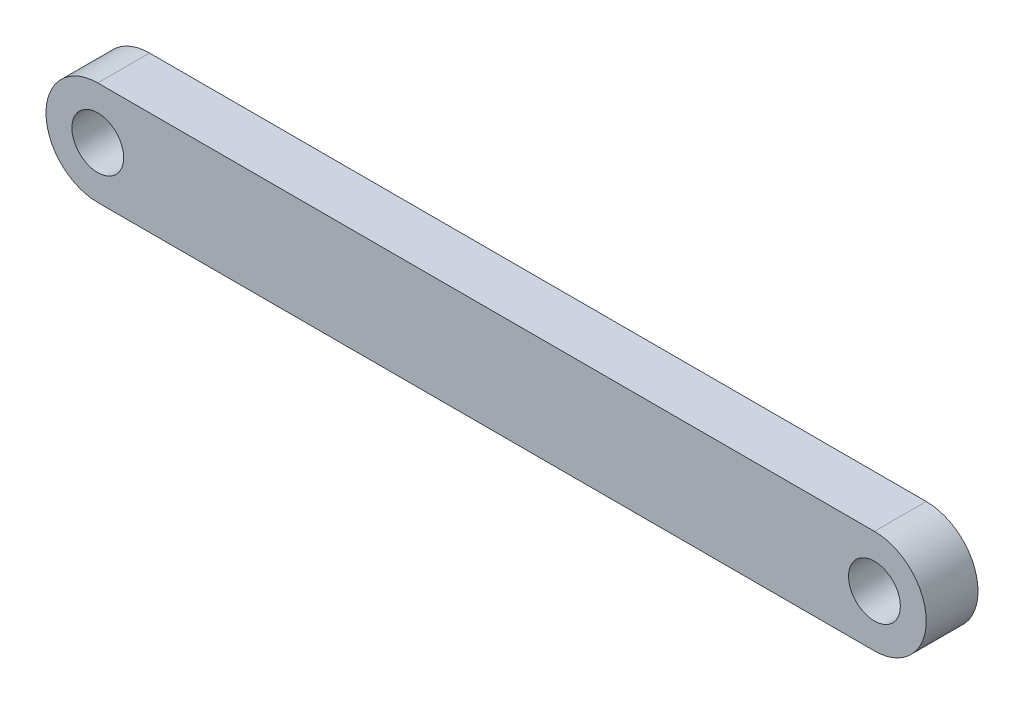
SolidWorks part; units mm, degrees
ref_plane "Front Plane" through (0, 0, 0) normal (0, 0, 1) x (1, 0, 0)
ref_plane "Top Plane" through (0, 0, 0) normal (0, 1, 0) x (1, 0, 0)
ref_plane "Right Plane" through (0, 0, 0) normal (1, 0, 0) x (0, 0, -1)
other "Configuration Table"
sketch "Sketch1" plane through (0, 0, 0) normal (0, 0, 1) x (1, 0, 0)
  line L0 (0, 0) -> (45, 0) construction
  line L1 (0, 3) -> (45, 3)
  line L2 (0, -3) -> (45, -3)
  arc A0 (0, 3) -> (0, -3) centre (0, 0) ccw
  arc A1 (45, -3) -> (45, 3) centre (45, 0) ccw
  circle A2 centre (0, 0) radius 1.5
  circle A3 centre (45, 0) radius 1.5
  point P3 (22.5, 0)
  dimension "D3" = 3
  dimension "D1" = 45
  dimension "D2" = 6
extrude "Boss-Extrude1" add sketch "Sketch1" along normal blind 3
